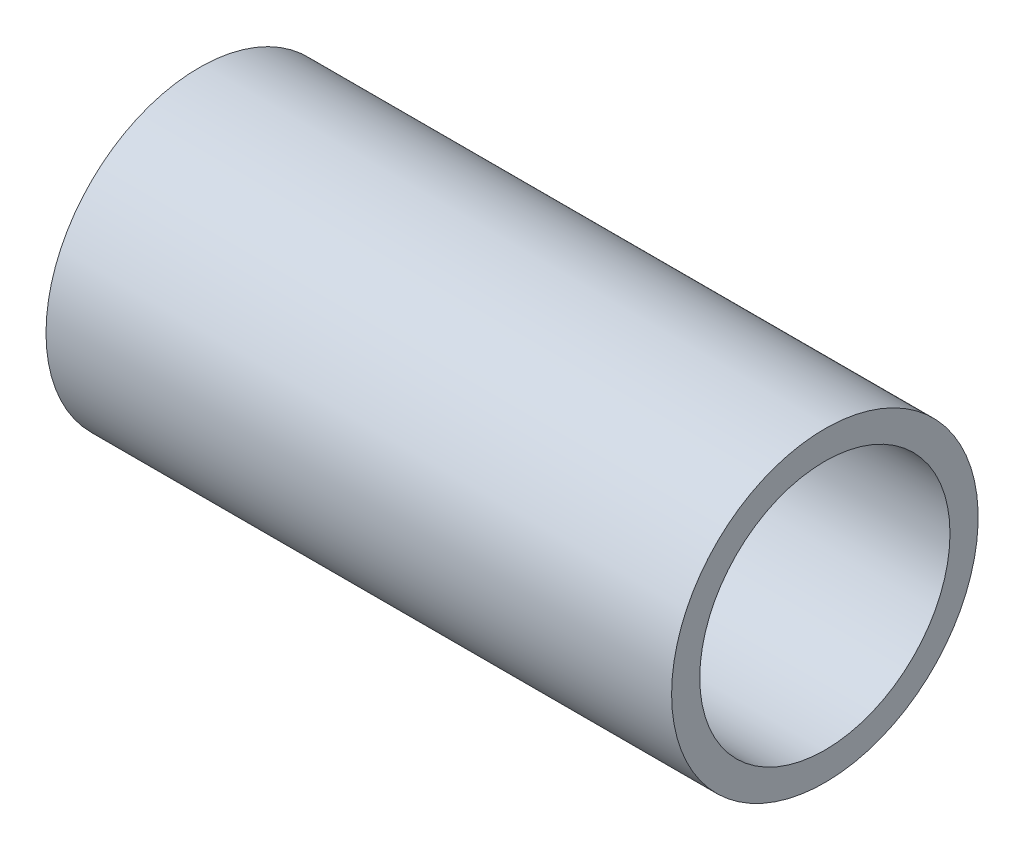
from build123d import *

# Parameters (mm, degrees)
SKETCH1_W = 20
SKETCH1_H = 0.9


with BuildPart() as part:
    # Sketch1 → Revolve1 (revolve)
    with BuildSketch(Plane.XY, mode=Mode.PRIVATE) as revolve1_sk:
        with Locations((0, 4.45)):
            Rectangle(SKETCH1_W, SKETCH1_H)
    revolve(revolve1_sk.sketch.rotate(Axis((10, 0, 0), (-1, 0, 0)), 270), axis=Axis((10, 0, 0), (-1, 0, 0)))


solid = part.part
